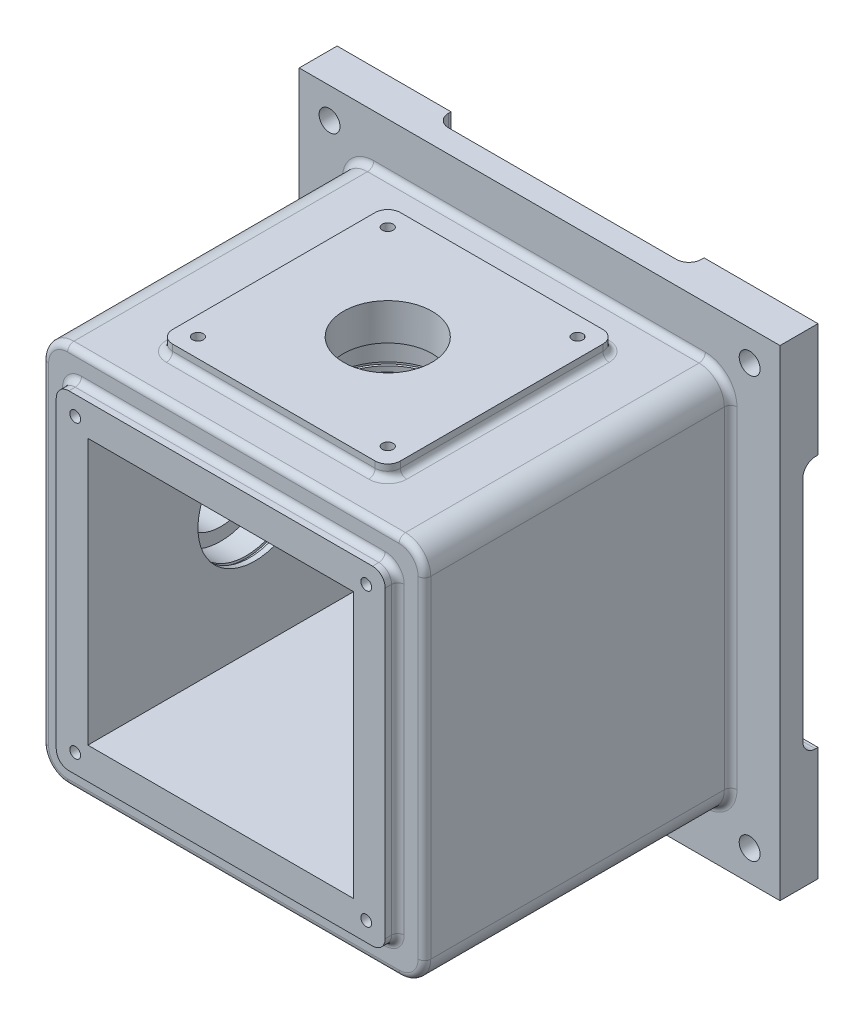
SolidWorks part; units mm, degrees
material "普通碳钢"
ref_plane "前视基准面" through (0, 0, 0) normal (0, 0, 1) x (1, 0, 0)
ref_plane "上视基准面" through (0, 0, 0) normal (0, 1, 0) x (1, 0, 0)
ref_plane "右视基准面" through (0, 0, 0) normal (1, 0, 0) x (0, 0, -1)
sketch "草图1" plane through (0, 0, 0) normal (0, 0, 1) x (1, 0, 0)
  line L1 (-190, 190) -> (190, 190)
  line L2 (-190, 190) -> (-190, -190)
  line L3 (-190, -190) -> (190, -190)
  line L4 (190, 190) -> (190, -190)
  line L5 (-190, 190) -> (190, -190) construction
  line L6 (-190, -190) -> (190, 190) construction
  line L7 (-166, -166) -> (166, -166) construction
  line L8 (-166, -166) -> (-166, 166) construction
  line L9 (-166, 166) -> (166, 166) construction
  line L10 (166, -166) -> (166, 166) construction
  line L11 (-166, -166) -> (166, 166) construction
  line L12 (-166, 166) -> (166, -166) construction
  circle A0 centre (-166, 166) radius 8.25
  circle A1 centre (166, 166) radius 8.25
  circle A2 centre (166, -166) radius 8.25
  circle A3 centre (-166, -166) radius 8.25
  point P0 (0, 0)
  point P6 (0, 0)
  dimension "D3" = 16.5
  dimension "D1" = 380
  dimension "D2" = 380
  dimension "D4" = 332
  dimension "D5" = 332
extrude "凸台-拉伸1" add sketch "草图1" along normal blind 30
sketch "草图2" plane through (0, -190, 0) normal (0, -1, 0) x (1, 0, 0)
  line L0 (0, 0) -> (0, 92.854) construction
  line L1 (-100, 0) -> (-100, 2)
  line L2 (-190, 0) -> (190, 0) construction
  line L3 (-90, 12) -> (90, 12)
  line L4 (100, 2) -> (100, 0)
  line L5 (100, 0) -> (-100, 0)
  arc A0 (90, 12) -> (100, 2) centre (90, 2) cw
  arc A1 (-100, 2) -> (-90, 12) centre (-90, 2) cw
  point P11 (100, 12)
  point P14 (-100, 12)
  dimension "D3" = 10
  dimension "D1" = 12
  dimension "D2" = 200
extrude "切除-拉伸1" cut sketch "草图2" against normal through all
sketch "草图3" plane through (190, 0, 0) normal (1, 0, 0) x (0, 0, -1)
  line L0 (0, 0) -> (-103.2239, 0) construction
  line L1 (0, -100) -> (-2, -100)
  line L2 (0, -190) -> (0, 190) construction
  line L3 (-12, -90) -> (-12, 90)
  line L4 (-2, 100) -> (0, 100)
  line L5 (0, 100) -> (0, -100)
  arc A0 (-12, 90) -> (-2, 100) centre (-2, 90) cw
  arc A1 (-2, -100) -> (-12, -90) centre (-2, -90) cw
  point P11 (-12, 100)
  point P14 (-12, -100)
  dimension "D3" = 10
  dimension "D1" = 200
  dimension "D2" = 12
extrude "切除-拉伸2" cut sketch "草图3" against normal through all
sketch "草图4" plane through (0, 0, 30) normal (0, 0, 1) x (1, 0, 0)
  line L1 (-131, 151) -> (131, 151)
  line L2 (-151, 131) -> (-151, -131)
  line L3 (-131, -151) -> (131, -151)
  line L4 (151, 131) -> (151, -131)
  line L5 (-151, 151) -> (151, -151) construction
  line L6 (-151, -151) -> (151, 151) construction
  arc A0 (-151, -131) -> (-131, -151) centre (-131, -131) ccw
  arc A1 (131, -151) -> (151, -131) centre (131, -131) ccw
  arc A2 (131, 151) -> (151, 131) centre (131, 131) cw
  arc A3 (-131, 151) -> (-151, 131) centre (-131, 131) ccw
  point P0 (0, 0)
  dimension "D3" = 20
  dimension "D1" = 302
  dimension "D2" = 302
extrude "凸台-拉伸2" add sketch "草图4" along normal blind 242
sketch "草图5" plane through (0, 151, 0) normal (0, 1, 0) x (1, 0, 0)
  line L0 (0, 0) -> (0, -340.7558) construction
  line L1 (0, 0) -> (-288.3435, 0) construction
  line L2 (80, -240) -> (-80, -240)
  line L3 (90, -230) -> (90, -70)
  line L4 (80, -60) -> (-80, -60)
  line L5 (-90, -230) -> (-90, -70)
  line L6 (90, -240) -> (-90, -60) construction
  line L7 (90, -60) -> (-90, -240) construction
  arc A0 (90, -70) -> (80, -60) centre (80, -70) ccw
  arc A1 (-80, -60) -> (-90, -70) centre (-80, -70) ccw
  arc A2 (-80, -240) -> (-90, -230) centre (-80, -230) cw
  arc A3 (80, -240) -> (90, -230) centre (80, -230) ccw
  point P3 (0, -150)
  dimension "D4" = 10
  dimension "D1" = 180
  dimension "D2" = 180
  dimension "D3" = 150
extrude "凸台-拉伸3" add sketch "草图5" along normal blind 10
sketch "草图7" plane through (0, 0, 272) normal (0, 0, 1) x (1, 0, 0)
  line L1 (-120, -130) -> (120, -130)
  line L2 (-130, -120) -> (-130, 120)
  line L3 (-120, 130) -> (120, 130)
  line L4 (130, -120) -> (130, 120)
  line L5 (-130, -130) -> (130, 130) construction
  line L6 (-130, 130) -> (130, -130) construction
  arc A0 (120, -130) -> (130, -120) centre (120, -120) ccw
  arc A1 (120, 130) -> (130, 120) centre (120, 120) cw
  arc A2 (-130, 120) -> (-120, 130) centre (-120, 120) cw
  arc A3 (-120, -130) -> (-130, -120) centre (-120, -120) cw
  point P0 (0, 0)
  dimension "D3" = 10
  dimension "D1" = 260
  dimension "D2" = 260
extrude "凸台-拉伸5" add sketch "草图7" along normal blind 10
sketch "草图8" plane through (0, 161, 0) normal (0, 1, 0) x (1, 0, 0)
  line L0 (0, 0) -> (0, -325.9411) construction
  line L1 (-90, -150) -> (90, -150) construction
  line L2 (-90, -70) -> (-90, -230) construction
  line L3 (90, -230) -> (90, -70) construction
  line L5 (75, -225) -> (-75, -225) construction
  line L6 (75, -225) -> (75, -75) construction
  line L7 (75, -75) -> (-75, -75) construction
  line L8 (-75, -225) -> (-75, -75) construction
  line L9 (75, -225) -> (-75, -75) construction
  line L10 (75, -75) -> (-75, -225) construction
  point P9 (0, -150)
  dimension "D1" = 150
  dimension "D2" = 150
hole_wizard "M10 螺纹孔1" positions "3D草图2" profile "草图9" tap size "M10" standard "GB"
sketch3d "3D草图2"
  point P0 (75, 161, 225)
  point P3 (-75, 161, 225)
  point P6 (-75, 161, 75)
  point P9 (75, 161, 75)
sketch "草图9" plane through (75, 161, 225) normal (1, 0, 0) x (0, 0, 1)
  line L0 (0, 0) -> (0, 24.5537)
  line L1 (0, 24.5537) -> (4.25, 22)
  line L2 (4.25, 22) -> (4.25, 0)
  line L5 (4.25, 0) -> (0, 0)
  line L10 (0, 24.5537) -> (-4.25, 22) construction
  line L11 (0, -6.35) -> (0, 107.95) construction
  dimension "螺纹孔钻头直径" = 8.5
  dimension "螺纹孔钻头深度" = 22
  dimension "导头角度" = 118
cosmetic thread "孔螺蚊线1" parameters "D1"=20, "D2"=10
cosmetic thread "孔螺蚊线2" parameters "D1"=20, "D2"=10
cosmetic thread "孔螺蚊线3" parameters "D1"=20, "D2"=10
cosmetic thread "孔螺蚊线4" parameters "D1"=20, "D2"=10
sketch "草图12" plane through (0, 0, 282) normal (0, 0, 1) x (1, 0, 0)
  line L1 (115, 115) -> (-115, 115) construction
  line L2 (115, 115) -> (115, -115) construction
  line L3 (115, -115) -> (-115, -115) construction
  line L4 (-115, 115) -> (-115, -115) construction
  line L5 (115, 115) -> (-115, -115) construction
  line L6 (115, -115) -> (-115, 115) construction
  point P0 (0, 0)
  point P1 (0, 0)
  dimension "D1" = 230
  dimension "D2" = 230
hole_wizard "M10 螺纹孔3" positions "3D草图4" profile "草图13" tap size "M10" standard "GB"
sketch3d "3D草图4"
  point P0 (115, -115, 282)
  point P3 (115, 115, 282)
  point P6 (-115, 115, 282)
  point P9 (-115, -115, 282)
sketch "草图13" plane through (115, -115, 282) normal (1, 0, 0) x (0, -1, 0)
  line L0 (0, 0) -> (0, 24.5537)
  line L1 (0, 24.5537) -> (4.25, 22)
  line L2 (4.25, 22) -> (4.25, 0)
  line L5 (4.25, 0) -> (0, 0)
  line L10 (0, 24.5537) -> (-4.25, 22) construction
  line L11 (0, -6.35) -> (0, 107.95) construction
  dimension "螺纹孔钻头直径" = 8.5
  dimension "螺纹孔钻头深度" = 22
  dimension "导头角度" = 118
cosmetic thread "孔螺蚊线9" parameters "D1"=20, "D2"=10
cosmetic thread "孔螺蚊线10" parameters "D1"=20, "D2"=10
cosmetic thread "孔螺蚊线11" parameters "D1"=20, "D2"=10
cosmetic thread "孔螺蚊线12" parameters "D1"=20, "D2"=10
sketch "草图14" plane through (0, 0, 282) normal (0, 0, 1) x (1, 0, 0)
  line L1 (-105, -105) -> (105, -105)
  line L2 (-105, -105) -> (-105, 105)
  line L3 (-105, 105) -> (105, 105)
  line L4 (105, -105) -> (105, 105)
  line L5 (-105, -105) -> (105, 105) construction
  line L6 (-105, 105) -> (105, -105) construction
  point P0 (0, 0)
  dimension "D1" = 210
  dimension "D2" = 210
extrude "切除-拉伸3" cut sketch "草图14" against normal blind 252
sketch "草图15" plane through (-151, 0, 0) normal (-1, 0, 0) x (0, 0, 1)
  line L0 (0, 0) -> (339.8246, 0) construction
  circle A0 centre (150, 0) radius 90
  point P3 (150, 0)
  dimension "D1" = 180
  dimension "D3" = 150
extrude "凸台-拉伸6" add sketch "草图15" along normal blind 20
fillet "圆角1" radius 5 32 edges at (-127.0711, 127.0711, 272) (0, 130, 272) (127.0711, 127.0711, 272) (130, 0, 272) (127.0711, -127.0711, 272) (0, -130, 272) (-127.0711, -127.0711, 272) (-145.1421, 145.1421, 272) (0, 151, 272) (145.1421, 145.1421, 272) (151, 0, 272) (145.1421, -145.1421, 272) (0, -151, 272) (-145.1421, -145.1421, 272) (-87.0711, 151, 62.9289) (0, 151, 60) (87.0711, 151, 62.9289) (90, 151, 150) (87.0711, 151, 237.0711) (0, 151, 240) (-87.0711, 151, 237.0711) (145.1421, 145.1421, 30) (151, 0, 30) (145.1421, -145.1421, 30) (0, -151, 30) (-145.1421, -145.1421, 30) (-151, 0, 30) (-145.1421, 145.1421, 30) (-130, 0, 272) (-151, 0, 272) (-90, 151, 150) (0, 151, 30)
sketch "草图18" plane through (0, 161, 0) normal (0, 1, 0) x (1, 0, 0)
  line L0 (0, 0) -> (0, -292.809) construction
  line L1 (-90, -150) -> (90, -150) construction
  line L2 (-90, -70) -> (-90, -230) construction
  line L3 (90, -230) -> (90, -70) construction
  circle A0 centre (0, -150) radius 35
  dimension "D1" = 70
extrude "切除-拉伸4" cut sketch "草图18" against normal up to next
sketch "草图19" plane through (-171, 0, 0) normal (-1, 0, 0) x (0, 0, 1)
  line L0 (0, 0) -> (296.9904, 0) construction
  line L1 (150, -90) -> (150, 90) construction
  circle A0 centre (150, 0) radius 35
  dimension "D1" = 70
  dimension "D2" = 150
extrude "切除-拉伸5" cut sketch "草图19" against normal up to next
sketch "草图20" plane through (0, 105, 0) normal (0, -1, 0) x (1, 0, 0)
  circle A0 centre (0, 150) radius 45
  dimension "D1" = 90
extrude "切除-拉伸6" cut sketch "草图20" against normal blind 27
sketch "草图21" plane through (-105, 0, 0) normal (1, 0, 0) x (0, 0, -1)
  circle A0 centre (-150, 0) radius 45
  dimension "D1" = 90
extrude "切除-拉伸7" cut sketch "草图21" against normal blind 27
sketch "草图22" plane through (-171, 0, 0) normal (-1, 0, 0) x (0, 0, 1)
  line L0 (150, 0) -> (261.1578, 0) construction
  point P4 (225, 0)
  point P8 (187.5, -64.9519)
  point P9 (112.5, -64.9519)
  point P10 (75, 0)
  point P11 (112.5, 64.9519)
  point P12 (187.5, 64.9519)
  point P13 (150, 0)
  dimension "D1" = 75
  dimension "D2" = 6
hole_wizard "M10 螺纹孔4" positions "3D草图5" profile "草图23" tap size "M10" standard "GB"
sketch3d "3D草图5"
  point P0 (-171, 0, 225)
  point P3 (-171, -64.9519, 187.5)
  point P6 (-171, -64.9519, 112.5)
  point P9 (-171, 0, 75)
  point P12 (-171, 64.9519, 112.5)
  point P15 (-171, 64.9519, 187.5)
sketch "草图23" plane through (-171, 0, 225) normal (0, 1, 0) x (0, 0, 1)
  line L0 (0, 0) -> (0, 24.5537)
  line L1 (0, 24.5537) -> (4.25, 22)
  line L2 (4.25, 22) -> (4.25, 0)
  line L5 (4.25, 0) -> (0, 0)
  line L10 (0, 24.5537) -> (-4.25, 22) construction
  line L11 (0, -6.35) -> (0, 107.95) construction
  dimension "螺纹孔钻头直径" = 8.5
  dimension "螺纹孔钻头深度" = 22
  dimension "导头角度" = 118
cosmetic thread "孔螺蚊线13" parameters "D1"=20, "D2"=10
cosmetic thread "孔螺蚊线14" parameters "D1"=20, "D2"=10
cosmetic thread "孔螺蚊线15" parameters "D1"=20, "D2"=10
cosmetic thread "孔螺蚊线16" parameters "D1"=20, "D2"=10
cosmetic thread "孔螺蚊线17" parameters "D1"=20, "D2"=10
cosmetic thread "孔螺蚊线18" parameters "D1"=20, "D2"=10
fillet "圆角2" radius 5 1 edges at (-151, 90, 150)
ref_plane "基准面1" through (-112, 0, 0) normal (1, 0, 0) x (0, 0, -1)
sketch "草图24" plane through (-112, 0, 0) normal (1, 0, 0) x (0, 0, -1)
  circle A0 centre (-150, 0) radius 46.75
  dimension "D1" = 93.5
extrude "切除-拉伸8" cut sketch "草图24" along normal blind 2.7
ref_plane "基准面2" through (0, 112, 0) normal (0, -1, 0) x (-1, 0, 0)
sketch "草图25" plane through (0, 112, 0) normal (0, -1, 0) x (-1, 0, 0)
  circle A0 centre (0, -150) radius 46.75
  dimension "D1" = 93.5
extrude "切除-拉伸9" cut sketch "草图25" along normal blind 2.7
ref_plane "基准面3" through (0, 0, 150) normal (0, 0, 1) x (1, 0, 0)
